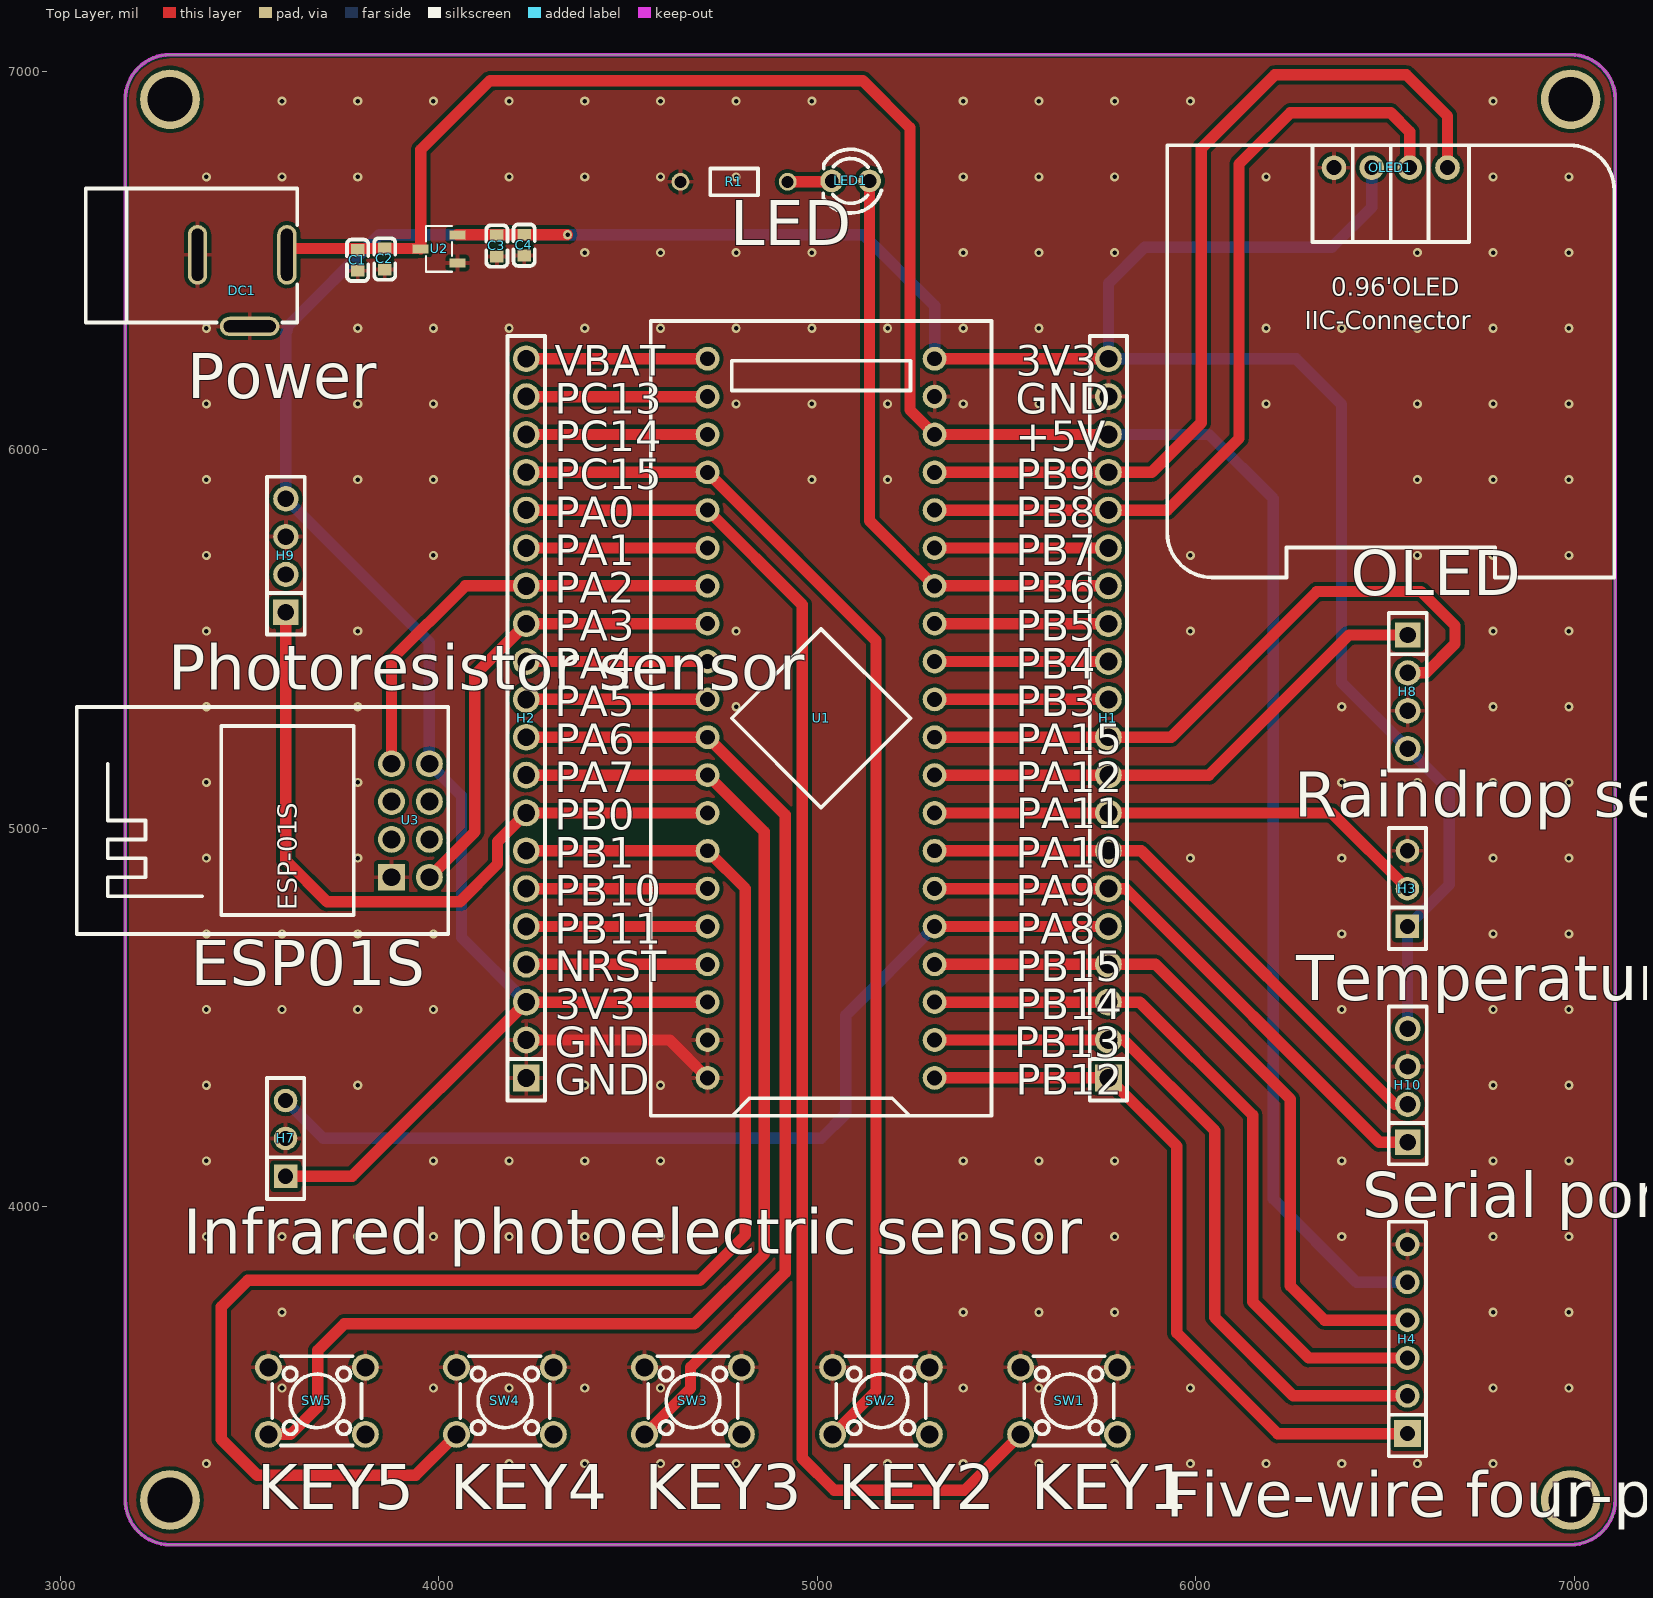
[diagram p0: Top Layer view]
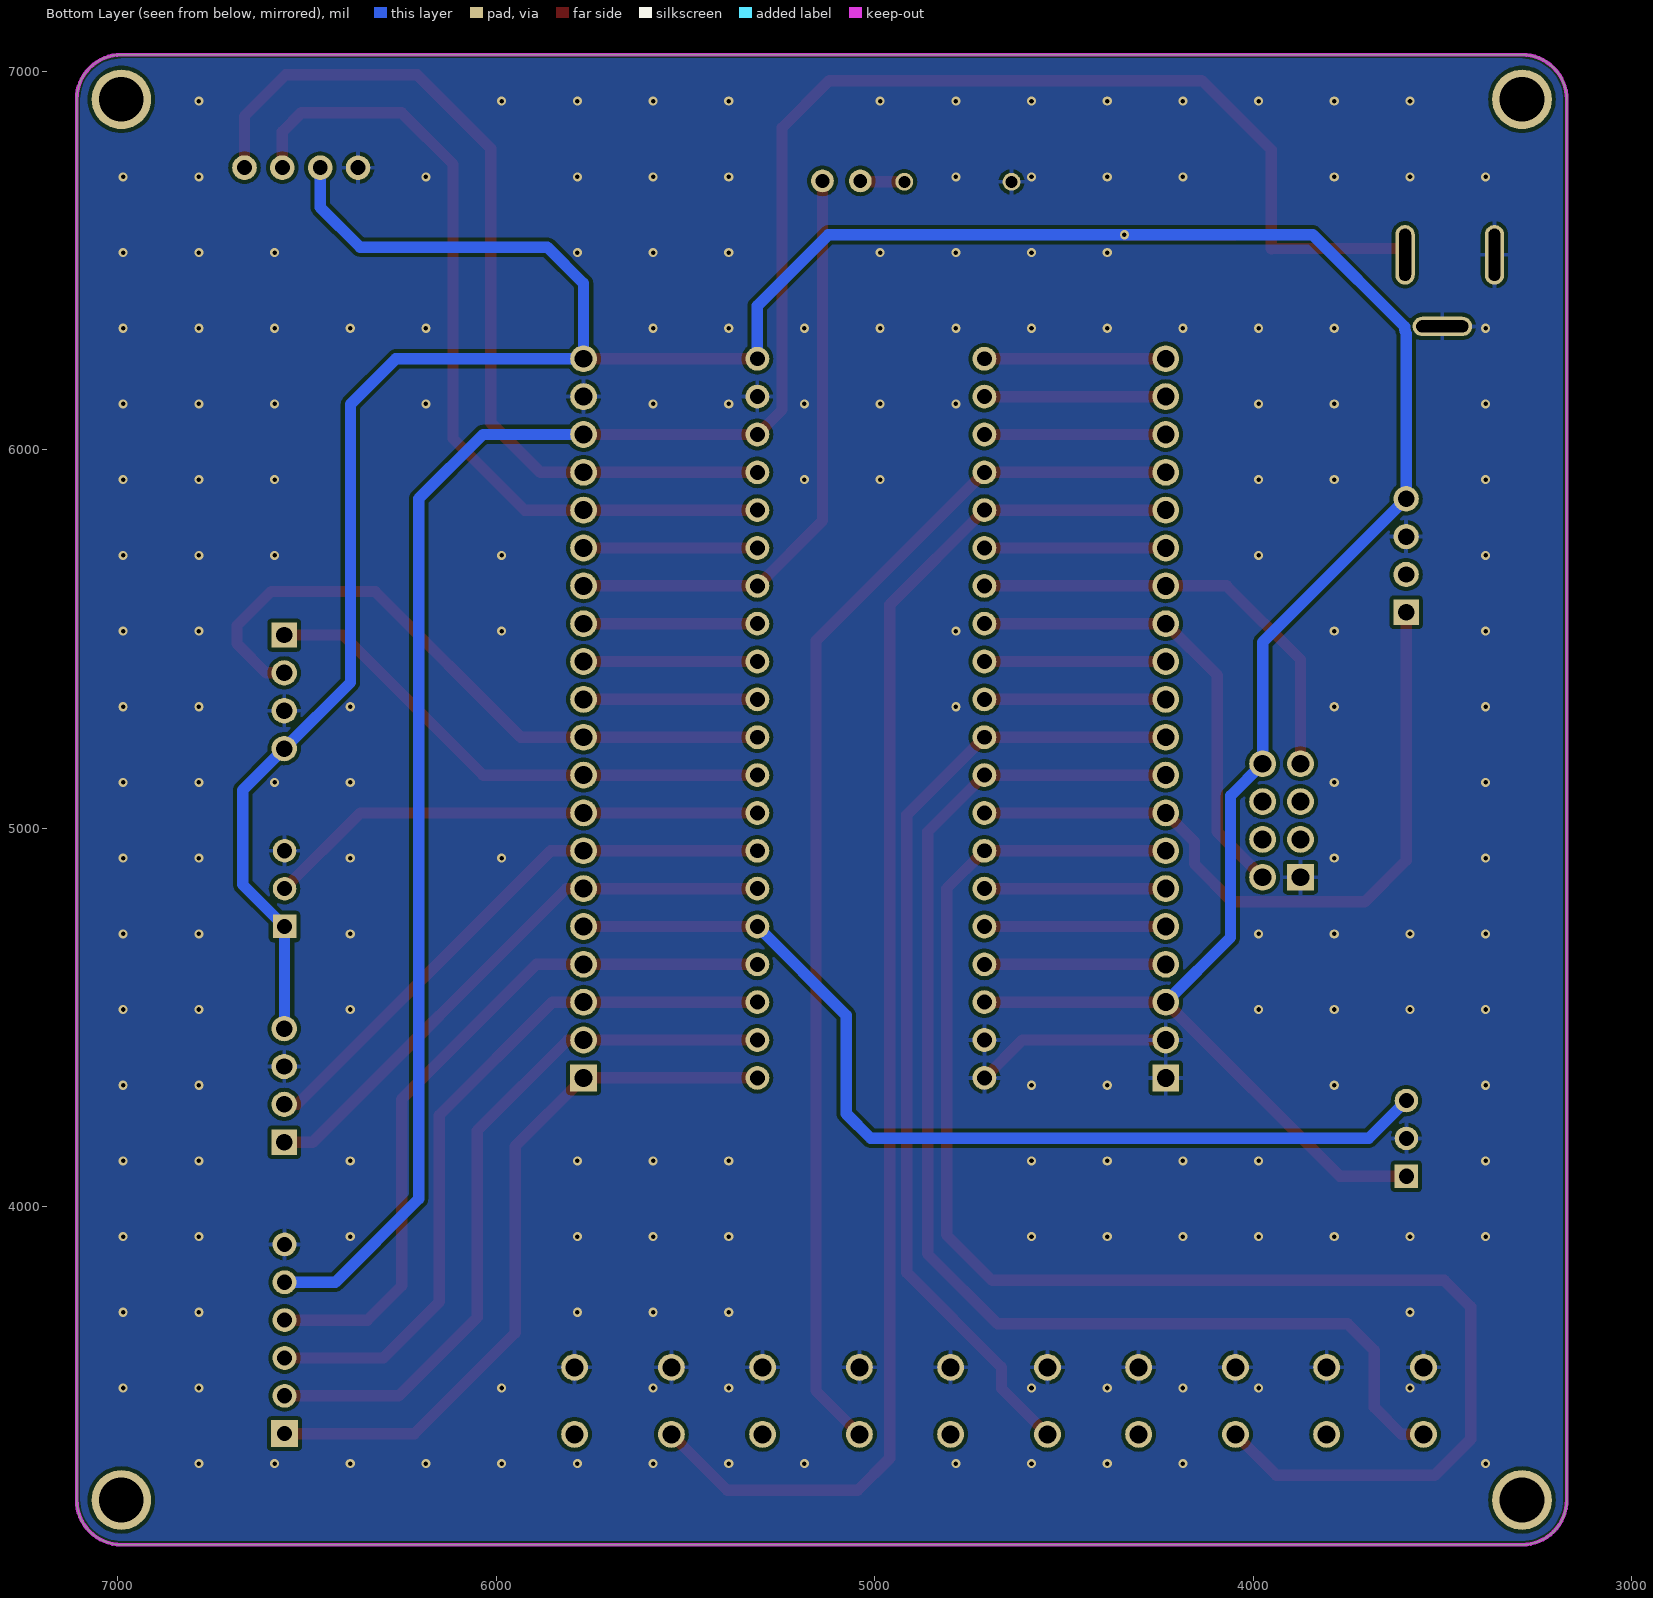
[diagram p1: Bottom Layer view, seen from below]
# Altium PCB MISC50760.pcbdoc
Units mil, origin at the board's own origin, x right, y up, seen from the top; angles counter-clockwise.
Board outline 3937.01 x 3937.01 mil, 2 copper layers (Top Layer, Bottom Layer), stack 62.206 mil thick; 24 components, 38 nets, 158 pads, 177 vias.

## Layer stack, top to bottom
Top Solder Mask Layer: solder mask 0.394, Dk 3.3
Top Layer: signal copper 1.379
Dielectric1: surface 59.449, FR4, Dk 4.5
Bottom Layer: signal copper 1.378
Bottom Solder Mask Layer: solder mask 0.394, Dk 3.3

## Board outline
3289.61,7043.5 ccw(c3289.61,6925.39) 3171.5,6925.39 3171.5,3224.61 ccw(c3289.61,3224.61) 3289.61,3106.5 6990.39,3106.5 ccw(c6990.39,3224.61) 7108.5,3224.61 7108.5,6925.39 ccw(c6990.39,6925.39) 6990.39,7043.5 3289.61,7043.5

## Design rules (kind name [scope] priority, off if disabled: settings)
BoardOutlineClearance copperThickness2oz_1 [All] p2 off: genericclearance=7.99 ignorepadtopadclearanceinfootprint=FALSE except(0: Arc-SplitContinuation Track-SplitContinuation SMDPad-SplitContinuation THPad-SplitContinuation Via-SplitContinuation Fill-SplitContinuation Region-SplitContinuation Poly-SplitContinuation Text-SplitContinuation Hole-SplitContinuation; 5.98: Arc-CutoutEdge Track-CutoutEdge SMDPad-CutoutEdge THPad-CutoutEdge Via-CutoutEdge Text-CutoutEdge; 6.9: Hole-OutlineEdge Hole-CutoutEdge; 10: Poly-OutlineEdge Poly-CutoutEdge; 11.81: Arc-OutlineEdge Track-OutlineEdge SMDPad-OutlineEdge THPad-OutlineEdge Via-OutlineEdge Fill-OutlineEdge Region-OutlineEdge Text-OutlineEdge Fill-CutoutEdge Region-CutoutEdge)
BoardOutlineClearance Plane_innerPlane_1 [All] p4 off: genericclearance=4.02 ignorepadtopadclearanceinfootprint=FALSE except(0: Arc-SplitContinuation Track-SplitContinuation SMDPad-SplitContinuation THPad-SplitContinuation Via-SplitContinuation Fill-SplitContinuation Region-SplitContinuation Poly-SplitContinuation Text-SplitContinuation Hole-SplitContinuation; 5.98: Arc-CutoutEdge Track-CutoutEdge SMDPad-CutoutEdge THPad-CutoutEdge Via-CutoutEdge Text-CutoutEdge; 6.9: Hole-OutlineEdge Hole-CutoutEdge; 10: Poly-OutlineEdge Poly-CutoutEdge; 11.81: Arc-OutlineEdge Track-OutlineEdge SMDPad-OutlineEdge THPad-OutlineEdge Via-OutlineEdge Fill-OutlineEdge Region-OutlineEdge Text-OutlineEdge Fill-CutoutEdge Region-CutoutEdge)
BoardOutlineClearance Copper_copperRegion_1 [All] p6 off: genericclearance=4.02 ignorepadtopadclearanceinfootprint=FALSE except(0: Arc-SplitContinuation Track-SplitContinuation SMDPad-SplitContinuation THPad-SplitContinuation Via-SplitContinuation Fill-SplitContinuation Region-SplitContinuation Poly-SplitContinuation Text-SplitContinuation Hole-SplitContinuation; 5.98: Arc-CutoutEdge Track-CutoutEdge SMDPad-CutoutEdge THPad-CutoutEdge Via-CutoutEdge Text-CutoutEdge; 6.9: Hole-OutlineEdge Hole-CutoutEdge; 10: Poly-OutlineEdge Poly-CutoutEdge; 11.81: Arc-OutlineEdge Track-OutlineEdge SMDPad-OutlineEdge THPad-OutlineEdge Via-OutlineEdge Fill-OutlineEdge Region-OutlineEdge Text-OutlineEdge Fill-CutoutEdge Region-CutoutEdge)
BoardOutlineClearance copperThickness1oz_1 [All] p8: genericclearance=4.02 ignorepadtopadclearanceinfootprint=FALSE except(0: Arc-SplitContinuation Track-SplitContinuation SMDPad-SplitContinuation THPad-SplitContinuation Via-SplitContinuation Fill-SplitContinuation Region-SplitContinuation Poly-SplitContinuation Text-SplitContinuation Hole-SplitContinuation; 5.98: Arc-CutoutEdge Track-CutoutEdge SMDPad-CutoutEdge THPad-CutoutEdge Via-CutoutEdge Text-CutoutEdge; 6.9: Hole-OutlineEdge Hole-CutoutEdge; 10: Poly-OutlineEdge Poly-CutoutEdge; 11.81: Arc-OutlineEdge Track-OutlineEdge SMDPad-OutlineEdge THPad-OutlineEdge Via-OutlineEdge Fill-OutlineEdge Region-OutlineEdge Text-OutlineEdge Fill-CutoutEdge Region-CutoutEdge)
Clearance copperThickness2oz [All] p1 off: gap=7.99 ignorepadtopadclearanceinfootprint=FALSE except(5.98: SMDPad-Track SMDPad-SMDPad THPad-Track SMDPad-THPad THPad-THPad Track-Via SMDPad-Via THPad-Via Via-Via Fill-SMDPad Region-SMDPad Fill-THPad Region-THPad Fill-Via Region-Via Fill-Fill Fill-Region Region-Region Arc-Track Arc-SMDPad Arc-THPad Arc-Via Fill-Arc Region-Arc Arc-Arc Text-Track SMDPad-Text Text-THPad Text-Via Fill-Text Region-Text Arc-Text Text-Text; 6.9: Hole-Track Hole-SMDPad Hole-THPad Hole-Via Fill-Hole Region-Hole Hole-Arc Hole-Text; 10: Poly-Track Poly-SMDPad Poly-THPad Poly-Via Poly-Fill Poly-Region Poly-Poly Poly-Arc Poly-Text Poly-Hole; 11.81: Fill-Track Region-Track)
Clearance Plane_innerPlane [All] p3 off: gap=4.02 ignorepadtopadclearanceinfootprint=FALSE except(5.98: SMDPad-Track SMDPad-SMDPad THPad-Track SMDPad-THPad THPad-THPad Track-Via SMDPad-Via THPad-Via Via-Via Fill-SMDPad Region-SMDPad Fill-THPad Region-THPad Fill-Via Region-Via Fill-Fill Fill-Region Region-Region Arc-Track Arc-SMDPad Arc-THPad Arc-Via Fill-Arc Region-Arc Arc-Arc Text-Track SMDPad-Text Text-THPad Text-Via Fill-Text Region-Text Arc-Text Text-Text; 6.9: Hole-Track Hole-SMDPad Hole-THPad Hole-Via Fill-Hole Region-Hole Hole-Arc Hole-Text; 10: Poly-Track Poly-SMDPad Poly-THPad Poly-Via Poly-Fill Poly-Region Poly-Poly Poly-Arc Poly-Text Poly-Hole; 11.81: Fill-Track Region-Track)
Clearance Copper_copperRegion [All] p5 off: gap=4.02 ignorepadtopadclearanceinfootprint=FALSE except(5.98: SMDPad-Track SMDPad-SMDPad THPad-Track SMDPad-THPad THPad-THPad Track-Via SMDPad-Via THPad-Via Via-Via Fill-SMDPad Region-SMDPad Fill-THPad Region-THPad Fill-Via Region-Via Fill-Fill Fill-Region Region-Region Arc-Track Arc-SMDPad Arc-THPad Arc-Via Fill-Arc Region-Arc Arc-Arc Text-Track SMDPad-Text Text-THPad Text-Via Fill-Text Region-Text Arc-Text Text-Text; 6.9: Hole-Track Hole-SMDPad Hole-THPad Hole-Via Fill-Hole Region-Hole Hole-Arc Hole-Text; 10: Poly-Track Poly-SMDPad Poly-THPad Poly-Via Poly-Fill Poly-Region Poly-Poly Poly-Arc Poly-Text Poly-Hole; 11.81: Fill-Track Region-Track)
Clearance copperThickness1oz [All] p7: gap=4.02 ignorepadtopadclearanceinfootprint=FALSE except(5.98: SMDPad-Track SMDPad-SMDPad THPad-Track SMDPad-THPad THPad-THPad Track-Via SMDPad-Via THPad-Via Via-Via Fill-SMDPad Region-SMDPad Fill-THPad Region-THPad Fill-Via Region-Via Fill-Fill Fill-Region Region-Region Arc-Track Arc-SMDPad Arc-THPad Arc-Via Fill-Arc Region-Arc Arc-Arc Text-Track SMDPad-Text Text-THPad Text-Via Fill-Text Region-Text Arc-Text Text-Text; 6.9: Hole-Track Hole-SMDPad Hole-THPad Hole-Via Fill-Hole Region-Hole Hole-Arc Hole-Text; 10: Poly-Track Poly-SMDPad Poly-THPad Poly-Via Poly-Fill Poly-Region Poly-Poly Poly-Arc Poly-Text Poly-Hole; 11.81: Fill-Track Region-Track)
DiffPairsRouting differentialPair [All] p1: maxlimit=6 minlimit=6 mostfreqgap=6 toplayer_minwidth=5 toplayer_prefwidth=10 toplayer_maxwidth=100 toplayer_mingap=6 toplayer_prefgap=6 toplayer_maxgap=6 bottomlayer_minwidth=5 bottomlayer_prefwidth=10 bottomlayer_maxwidth=100 bottomlayer_mingap=6 bottomlayer_prefgap=6 bottomlayer_maxgap=6 maxuncoupledlength=10
HoleToHoleClearance otherClearance [All] p1: gap=11.81 allowstackedmicrovias=TRUE
Length netLength [All] p1: minlimit=0 maxlimit=0
PasteMaskExpansion pasteMaskExpansion [All] p1: expansion=0
PlaneConnect innerPlane [All] p1: planeconnectstyle=Relief reliefexpansion=20 reliefentries=4 reliefconductorwidth=10 reliefairgap=10
PolygonConnect copperRegion [All] p1: connectstyle=Relief reliefconductorwidth=10 reliefentries=4 polygonreliefangle="90 Angle" airgapwidth=10 via.connectstyle=Relief via.reliefconductorwidth=10 via.reliefentries=4 via.polygonreliefangle="90 Angle" via.airgapwidth=10
RoutingVias viaSize [All] p1: holewidth=12.01 width=24.02 viastyle="Through Hole" minholewidth=11.81 minwidth=19.68 maxholewidth=248.03 maxwidth=393.7
SolderMaskExpansion solderMaskExpansion [IsVia] p1: expansion=-1000 istentingtop=TRUE
SolderMaskExpansion solderMaskExpansion [All] p2: expansion=2 istentingtop=FALSE
Width copperThickness2oz_2 [All] p1 off: maxlimit=100 minlimit=8 preferedwidth=10
Width copperThickness1oz_2 [All] p2: maxlimit=100 minlimit=5 preferedwidth=10

## Components (designator, comment, footprint, x,y, rotation, side; value= is the part's Value field where it differs from the comment)
C1 "10uF" C0603 3785.45,6500.1 r90 top
C2 "100nF" C0603 3856.99,6503.61 r90 top
C3 "10uF" C0603 4153.37,6538.01 r90 top
C4 "100nF" C0603 4225.45,6540.1 r90 top
DC1 "" DC-2.0 3475.44,6525.1 r180 top
H1 "" HDR-TH_20P-P2.54-V-F 5769.16,5290 r90 top
H2 "" HDR-TH_20P-P2.54-V-F 4230.95,5290 r90 top
H3 "" HDR-TH_3P-P2.54-V-F 6559.21,4840 r90 top
H4 "" HDR-TH_6P-P2.54-V-F 6559.21,3650 r90 top
H7 "" HDR-TH_3P-P2.54-V-F 3595,4180 r90 top
H8 "" HDR-TH_4P-P2.54-V-F 6560,5360 r270 top
H9 "" HDR-TH_4P-P2.54-V-F 3595.79,5720 r90 top
H10 "" HDR-TH_4P-P2.54-V-F 6560,4320 r90 top
LED1 "" LED_TH-3mm 5087.95,6709.8 r180 top
OLED1 "" 0.96OLED_4P 6515,6745 r0 top
R1 "220" Res_1/8W 4780,6710 r180 top
SW1 "" SW-TH_4P-L6.0-W6.0-P4.50-LS6.5 5665,3486.58 r0 top
SW2 "" SW-TH_4P-L6.0-W6.0-P4.50-LS6.5 5168.22,3486.58 r0 top
SW3 "" SW-TH_4P-L6.0-W6.0-P4.50-LS6.5 4671.43,3486.58 r0 top
SW4 "" SW-TH_4P-L6.0-W6.0-P4.50-LS6.5 4174.65,3486.58 r0 top
SW5 "" SW-TH_4P-L6.0-W6.0-P4.50-LS6.5 3677.86,3486.58 r0 top
U1 "STM32F103C8T6-Card" CONN-TH_L53.3-W22.9_STM32F103C8T6-CARD 5010,5290 r90 top
U2 "HT7333" SOT-23-3_L2.9-W1.6-P1.90-LS2.8-BR 4000.45,6530.1 r0 top
U3 "ESP-01S" WIFIM-TH_ESP-01S 3925,5020 r90 top

## Footprints (in the part's own frame and the unit in brackets; to place one, negate y for a bottom-side part, rotate by r counter-clockwise, add the part's x,y. Pads: shape width x height; smd on the part's side, far side on the other; paste and mask are expansions set on the pad)
0.96OLED_4P [mm]
  round 1.65 hole 1 copper offset 0,0: 1(-3.81,-0.001) 2(-1.27,0.002) 3(1.27,0.002) 4(3.81,0.002)
  silkscreen extent -15,-27.5 15,1.5
C0603 [mm]
  rect 0.8x0.9 smd: 1(-0.7,0) 2(0.7,0)
  silkscreen extent -1.39,-0.71 1.39,0.71
CONN-TH_L53.3-W22.9_STM32F103C8T6-CARD [mm]
  round 1.6 hole 1: 1(-24.13,-7.62) 2(-21.59,-7.62) 3(-19.05,-7.62) 4(-16.51,-7.62) 5(-13.97,-7.62) 6(-11.43,-7.62) 7(-8.89,-7.62) 8(-6.35,-7.62) 9(-3.81,-7.62) 10(-1.27,-7.62) 11(1.27,-7.62) 12(3.81,-7.62) 13(6.35,-7.62) 14(8.89,-7.62) 15(11.43,-7.62) 16(13.97,-7.62) 17(16.51,-7.62) 18(19.05,-7.62) 19(21.59,-7.62) 20(24.13,-7.62) 21(24.13,7.62) 22(21.59,7.62) 23(19.05,7.62) 24(16.51,7.62) 25(13.97,7.62) 26(11.43,7.62) 27(8.89,7.62) 28(6.35,7.62) 29(3.81,7.62) 30(1.27,7.62) 31(-1.27,7.62) 32(-3.81,7.62) 33(-6.35,7.62) 34(-8.89,7.62) 35(-11.43,7.62) 36(-13.97,7.62) 37(-16.51,7.62) 38(-19.05,7.62) 39(-21.59,7.62) 40(-24.13,7.62)
  silkscreen extent -26.67,-11.43 26.67,11.43
DC-2.0 [mil]
  oval 157.5x51.2 hole 31.5 slot 137.8 at 0 deg paste+0 mask+2: 2(-24.7,199.5)
  oval 51.2x157.5 hole 31.5 slot 137.8 at 90 deg paste+0 mask+2: 3(113.1,10.5) 4(-123.1,10.5)
  silkscreen extent -151,-165 408,190
HDR-TH_3P-P2.54-V-F [mil]
  rect 62x62 hole 40.16: 1(-100,0)
  round 62 hole 40.16: 2(0,0) 3(100,0)
  silkscreen extent -160,-49 160,49
HDR-TH_4P-P2.54-V-F [mm]
  rect 1.7x1.7 hole 1.1: 1(-3.81,0)
  round 1.7 hole 1.1: 2(-1.27,0) 3(1.27,0) 4(3.81,0)
  silkscreen extent -5.29,-1.27 5.29,1.27
HDR-TH_6P-P2.54-V-F [mm]
  rect 1.8x1.8 hole 1.02: 1(-6.35,0)
  round 1.6 hole 1.02: 2(-3.81,0) 3(-1.27,0) 4(1.27,0) 5(3.81,0) 6(6.35,0)
  silkscreen extent -7.87,-1.25 7.87,1.25
HDR-TH_20P-P2.54-V-F [mm]
  rect 1.8x1.8 hole 1.2: 1(-24.13,0)
  round 1.8 hole 1.2: 2(-21.59,0) 3(-19.05,0) 4(-16.51,0) 5(-13.97,0) 6(-11.43,0) 7(-8.89,0) 8(-6.35,0) 9(-3.81,0) 10(-1.27,0) 11(1.27,0) 12(3.81,0) 13(6.35,0) 14(8.89,0) 15(11.43,0) 16(13.97,0) 17(16.51,0) 18(19.05,0) 19(21.59,0) 20(24.13,0)
  silkscreen extent -25.65,-1.25 25.65,1.25
LED_TH-3mm [mil]
  round 60 hole 36 paste+0 mask+2: 1(-50,0) 2(50,0)
  silkscreen extent -81,-84 72,85
Res_1/8W [mil]
  round 47.2 hole 31.5 paste+0 mask+2: 1(-141.7,2.48) 2(141.7,2.48)
  silkscreen extent -63,-33 63,38
SOT-23-3_L2.9-W1.6-P1.90-LS2.8-BR [mm]
  rect 1.07x0.6 smd: 1(1.235,-0.95) 2(1.235,0.95) 3(-1.235,0)
  silkscreen extent -0.88,-1.54 0.88,1.54
SW-TH_4P-L6.0-W6.0-P4.50-LS6.5 [mm]
  round 1.8 hole 1.2: 1(-3.25,2.25) 2(3.25,2.25) 3(-3.25,-2.25) 4(3.25,-2.25)
  silkscreen extent -3,-3 3,3
WIFIM-TH_ESP-01S [mm]
  rect 1.8x1.8 hole 1.2: 1(-3.81,1.27)
  round 1.8 hole 1.2: 2(-1.27,1.27) 3(1.27,1.27) 4(3.81,1.27) 5(3.81,-1.27) 6(1.27,-1.27) 7(-1.27,-1.27) 8(-3.81,-1.27)
  silkscreen extent -7.62,-2.54 7.62,22.4

## Free pads (board coordinates)
  round 157.48 hole 118.11: 1(3289.61,6925.39) 1(3289.61,3224.61) 1(6990.39,6925.39) 1(6990.39,3224.61)

## Via types
v1: diameter 24.02, hole 12, Top Layer to Bottom Layer, 177 vias

## Nets (pads, with @x,y where several pads share a name; then routed paths per layer and width w, separated by ;. In a path a pad name is that pad's centre, name@x,y a point inside that pad or via, vN(x,y) a via of type N, cw(c..) or ccw(c..) an arc to the next point about the centre after c; other vN are vias at no path point)
$1N17011: LED1.2 R1.1 | length 117.2
  Top Layer w30: R1.1 5035.67,6707.52 LED1.2
+5V: C1.2 C2.2 DC1.4 H1.18 H4.5 U1.18 U2.3 | length 6140.8
  Top Layer w30: DC1.4 3615.11,6531.17 C2.2 3950.75,6531.17 U2.3 3951.82,6791.82 4135,6975 5120,6975 5245,6850 5245,6105 U1.18 H1.18
  Bottom Layer w30: H1.18 6035,6040 6205,5870 6205,4020 6425,3800 H4.5
GND: C1.1 C2.1 C3.1 C4.1 DC1.2 DC1.3 H1.19 H2.1 H2.2 H3.3 H4.6 H7.2 H8.3 H9.3 H10.3 OLED1.1 R1.2 SW1.1 SW1.2 SW2.1 SW2.2 SW3.1 SW3.2 SW4.1 SW4.2 SW5.1 SW5.2 U1.19 U1.39 U1.40 U2.1 U3.1 | length 520.5
  Top Layer w30: H2.2 4610,4440 U1.40
  other v1: 3385.6,3320.6 4185.6,3320.6 4385.6,3320.6 4585.6,3320.6 4785.6,3320.6 5185.6,3320.6 5385.6,3320.6 5585.6,3320.6 5785.6,3320.6 5985.6,3320.6 6185.6,3320.6 6385.6,3320.6 6585.6,3320.6 6785.6,3320.6 3585.6,3520.6 3985.6,3520.6 4185.6,3520.6 4385.6,3520.6 4585.6,3520.6 5385.6,3520.6 5585.6,3520.6 5985.6,3520.6 6785.6,3520.6 6985.6,3520.6 3585.6,3720.6 5385.6,3720.6 5585.6,3720.6 5785.6,3720.6 6785.6,3720.6 6985.6,3720.6 3385.6,3920.6 3585.6,3920.6 3785.6,3920.6 3985.6,3920.6 4185.6,3920.6 4385.6,3920.6 4585.6,3920.6 5385.6,3920.6 5585.6,3920.6 5785.6,3920.6 6385.6,3920.6 6785.6,3920.6 6985.6,3920.6 3385.6,4120.6 3985.6,4120.6 4185.6,4120.6 4385.6,4120.6 4585.6,4120.6 5385.6,4120.6 5585.6,4120.6 5785.6,4120.6 6385.6,4120.6 6785.6,4120.6 6985.6,4120.6 3385.6,4320.6 3785.6,4320.6 4385.6,4320.6 4585.6,4320.6 6785.6,4320.6 6985.6,4320.6 3385.6,4520.6 3585.6,4520.6 3785.6,4520.6 3985.6,4520.6 6385.6,4520.6 6785.6,4520.6 6985.6,4520.6 3385.6,4720.6 3585.6,4720.6 3785.6,4720.6 3985.6,4720.6 6385.6,4720.6 6785.6,4720.6 6985.6,4720.6 3385.6,4920.6 3785.6,4920.6 5985.6,4920.6 6385.6,4920.6 6785.6,4920.6 6985.6,4920.6 3385.6,5120.6 3785.6,5120.6 6385.6,5120.6 6585.6,5120.6 6785.6,5120.6 6985.6,5120.6 3385.6,5320.6 3785.6,5320.6 4785.6,5320.6 6385.6,5320.6 6785.6,5320.6 6985.6,5320.6 3385.6,5520.6 3785.6,5520.6 4785.6,5520.6 5985.6,5520.6 6785.6,5520.6 6985.6,5520.6 3385.6,5720.6 3985.6,5720.6 5985.6,5720.6 6585.6,5720.6 6785.6,5720.6 6985.6,5720.6 3385.6,5920.6 3785.6,5920.6 3985.6,5920.6 4985.6,5920.6 5185.6,5920.6 6585.6,5920.6 6785.6,5920.6 6985.6,5920.6 3385.6,6120.6 3785.6,6120.6 3985.6,6120.6 4785.6,6120.6 4985.6,6120.6 5185.6,6120.6 5385.6,6120.6 5585.6,6120.6 6185.6,6120.6 6585.6,6120.6 6785.6,6120.6 6985.6,6120.6 3385.6,6320.6 3785.6,6320.6 3985.6,6320.6 4185.6,6320.6 4385.6,6320.6 4585.6,6320.6 4785.6,6320.6 4985.6,6320.6 5185.6,6320.6 5385.6,6320.6 5585.6,6320.6 6185.6,6320.6 6385.6,6320.6 6585.6,6320.6 6785.6,6320.6 6985.6,6320.6 4385.6,6520.6 4585.6,6520.6 4785.6,6520.6 4985.6,6520.6 5385.6,6520.6 5585.6,6520.6 5785.6,6520.6 6585.6,6520.6 6785.6,6520.6 6985.6,6520.6 3385.6,6720.6 3585.6,6720.6 3785.6,6720.6 4185.6,6720.6 4385.6,6720.6 4585.6,6720.6 4785.6,6720.6 5385.6,6720.6 5585.6,6720.6 5785.6,6720.6 6185.6,6720.6 6785.6,6720.6 6985.6,6720.6 3585.6,6920.6 3785.6,6920.6 3985.6,6920.6 4185.6,6920.6 4385.6,6920.6 4585.6,6920.6 4785.6,6920.6 4985.6,6920.6 5385.6,6920.6 5585.6,6920.6 5785.6,6920.6 5985.6,6920.6 6785.6,6920.6
NRST: H2.4 U1.37 | length 479
  Top Layer w30: H2.4 U1.37
PA0: H2.16 SW1.3 U1.25 | length 3761.2
  Top Layer w30: H2.16 U1.25 4960,5590 4960,3335 5045,3250 5389.05,3250 SW1.3
PA1: H2.15 U1.26 | length 479
  Top Layer w30: H2.15 U1.26
PA2: H2.14 U1.27 U3.4 | length 1190.8
  Top Layer w30: U3.4 3875,5445 4070,5640 H2.14 U1.27
PA3: H2.13 U1.28 U3.8 | length 1255.1
  Top Layer w30: U3.8 4095,4990 4095,5404.05 H2.13 U1.28
PA4: H2.12 U1.29 | length 479
  Top Layer w30: H2.12 U1.29
PA5: H2.11 U1.30 | length 479
  Top Layer w30: H2.11 U1.30
PA6: H2.10 SW3.3 U1.31 | length 2559.9
  Top Layer w30: H2.10 U1.31 4915,5035 4915,3825 4665,3575 4665,3519.52 SW3.3
PA7: H2.9 SW5.3 U1.32 | length 3401.7
  Top Layer w30: SW5.3 3608,3398 3680,3470 3680,3620 3750,3690 4675,3690 4860,3875 4860,4990 U1.32 H2.9
PA8: H1.5 H7.3 U1.5 | length 2599.8
  Top Layer w30: U1.5 H1.5
  Bottom Layer w30: H7.3 3695,4180 5010,4180 5075,4245 5075,4505 U1.5
PA9: H1.6 H10.1 U1.6 | length 1527.5
  Top Layer w30: U1.6 H1.6 5814.59,4840 6484.59,4170 H10.1
PA10: H1.7 H10.2 U1.7 | length 1527.5
  Top Layer w30: U1.7 H1.7 5856.01,4940 6526.01,4270 H10.2
PA11: H1.8 H3.2 U1.8 | length 1332.1
  Top Layer w30: U1.8 H1.8 6359.21,5040 H3.2
PA12: H1.9 H8.1 U1.9 | length 1403.3
  Top Layer w30: U1.9 H1.9 6035,5140 6405,5510 H8.1
PA15: H1.10 H8.2 U1.10 | length 1776.7
  Top Layer w30: U1.10 H1.10 5935,5240 6320,5625 6595,5625 6685,5535 6685,5486.89 6608.11,5410 H8.2
PB0: H2.8 H9.1 U1.33 | length 1947.2
  Top Layer w30: H9.1 3595.79,4914.21 3705,4805 4055,4805 4155,4905 4155,4964.05 H2.8 U1.33
PB1: H2.7 SW4.3 U1.34 | length 4055
  Top Layer w30: SW4.3 3938.7,3290 3520,3290 3425,3385 3425,3735 3495,3805 4690,3805 4810,3925 4810,4840 U1.34 H2.7
PB3: H1.11 U1.11 | length 459.2
  Top Layer w30: U1.11 H1.11
PB4: H1.12 U1.12 | length 459.2
  Top Layer w30: U1.12 H1.12
PB5: H1.13 U1.13 | length 459.2
  Top Layer w30: U1.13 H1.13
PB6: H1.14 LED1.1 U1.14 | length 1600.2
  Top Layer w30: LED1.1 5137.95,5812.05 U1.14 H1.14
PB7: H1.15 U1.15 | length 459.2
  Top Layer w30: U1.15 H1.15
PB8: H1.16 OLED1.3 U1.16 | length 2230.3
  Top Layer w30: U1.16 H1.16 5925,5840 6114.29,6029.29 6114.29,6754.29 6250,6890 6515,6890 6565,6840 OLED1.3@6565,6745.05
PB9: H1.17 OLED1.4 U1.17 | length 2396
  Top Layer w30: U1.17 H1.17 5883.58,5940 6014.29,6070.71 6014.29,6795.71 6208.58,6990 6556.42,6990 6665,6881.42 OLED1.4@6665,6745.05
PB10: H2.6 U1.35 | length 479
  Top Layer w30: H2.6 U1.35
PB11: H2.5 U1.36 | length 479
  Top Layer w30: H2.5 U1.36
PB12: H1.1 H4.1 U1.1 | length 1927.6
  Top Layer w30: U1.1 H1.1 5950,4159.16 5950,3665.74 6215.74,3400 H4.1
PB13: H1.2 H4.2 U1.2 | length 1927.6
  Top Layer w30: U1.2 H1.2 5810.58,4440 6050,4200.58 6050,3707.16 6257.16,3500 H4.2
PB14: H1.3 H4.3 U1.3 | length 1927.6
  Top Layer w30: U1.3 H1.3 5852,4540 6150,4242 6150,3748.58 6298.58,3600 H4.3
PB15: H1.4 H4.4 U1.4 | length 1927.6
  Top Layer w30: U1.4 H1.4 5893.42,4640 6250,4283.42 6250,3790 6340,3700 H4.4
PC13: H2.19 U1.22 | length 479
  Top Layer w30: H2.19 U1.22
PC14: H2.18 U1.23 | length 479
  Top Layer w30: H2.18 U1.23
PC15: H2.17 SW2.3 U1.24 | length 3252.9
  Top Layer w30: H2.17 U1.24 5155,5495 5155,3512.73 SW2.3
VBAT: H2.20 U1.21 | length 479
  Top Layer w30: H2.20 U1.21
VCC: C3.2 C4.2 H1.20 H2.3 H3.1 H7.1 H8.4 H9.4 H10.4 OLED1.2 U1.20 U1.38 U2.2 U3.5 | length 9695.7
  Top Layer w30: H7.1 3770.95,4080 H2.3 U1.38 ; U2.2 4225.29,6567.5 C4.2 v1(4340,6567.66) ; U1.20 H1.20
  Bottom Layer w30: H2.3 4060,4710.95 4060,5085 U3.5 3975,5490.79 H9.4 3595.79,6306.51 ccw(c3553.29,6325.6) 3599.87,6324.87 3842.66,6567.66 v1(4340,6567.66) 5122.34,6567.66 5310,6380 U1.20 ; OLED1.2@6465,6745.05 6465,6640 6360,6535 5865,6535 5769.16,6439.16 H1.20 6265,6240 6385,6120 6385,5385 H8.4 6670,5100 6670,4850.79 H3.1 6559.21,4470.79 H10.4
pads on no net: H9.2 SW1.4 SW2.4 SW3.4 SW4.4 SW5.4 U3.2 U3.3 U3.6 U3.7

## Polygon pours and split planes (outlines as drawn)
GND on Bottom Layer (solid, remove dead copper, pour order 2): 3100,7165 3100,3000 7275,3000 7275,7165
GND on Top Layer (solid, remove dead copper, pour order 0): 3000,7145 3000,3075 7385,3075 7385,7145

## Keep-outs
Board Outline Layer:
  the board outline again, w10

## Silkscreen, mask and mechanical layers (free items; w line width, h text height)
Top Silkscreen Layer:
  text "LED" at 4770,6540 h120
  text "VBAT" at 4305.95,6195 h80
  text "3V3" at 5524.16,6195 h80
  text "Power" at 3335,6135 h120
  text "PC13" at 4305.95,6095 h80
  text "GND" at 5524.16,6095 h80
  text "PC14" at 4305.95,5995 h80
  text "+5V" at 5524.16,5995 h80
  text "PC15" at 4305.95,5895 h80
  text "PB9" at 5524.16,5895 h80
  text "PA0" at 4305.95,5795 h80
  text "PB8" at 5524.16,5795 h80
  text "PA1" at 4305.95,5695 h80
  text "PB7" at 5524.16,5695 h80
  text "OLED" at 6410,5615 h120
  text "PA2" at 4305.95,5595 h80
  text "PB6" at 5524.16,5595 h80
  text "PA3" at 4305.95,5495 h80
  text "PB5" at 5524.16,5495 h80
  text "PA4" at 4305.95,5395 h80
  text "PB4" at 5524.16,5395 h80
  text "Photoresistor sensor" at 3285,5365 h120
  text "PA5" at 4305.95,5295 h80
  text "PB3" at 5524.16,5295 h80
  text "PA6" at 4305.95,5195 h80
  text "PA15" at 5524.16,5195 h80
  text "PA7" at 4305.95,5095 h80
  text "PA12" at 5524.16,5095 h80
  text "Raindrop sensor" at 6260,5030 h120
  text "PA11" at 5525.95,5000 h80
  text "PB0" at 4305.95,4995 h80
  text "PB1" at 4305.95,4895 h80
  text "PA10" at 5524.16,4895 h80
  text "PB10" at 4305.95,4795 h80
  text "PA9" at 5524.16,4795 h80
  text "PB11" at 4305.95,4695 h80
  text "PA8" at 5524.16,4695 h80
  text "NRST" at 4305.95,4595 h80
  text "PB15" at 5524.16,4595 h80
  text "ESP01S" at 3345,4585 h120
  text "Temperature and humidity sensor" at 6265,4545 h120
  text "3V3" at 4305.95,4495 h80
  text "PB14" at 5524.16,4495 h80
  text "GND" at 4305.95,4395 h80
  text "PB13" at 5520.95,4395 h80
  text "GND" at 4305.95,4295 h80
  text "PB12" at 5524.16,4295 h80
  text "Serial port" at 6439.21,3972.37 h120
  text "Infrared photoelectric sensor" at 3325,3875 h120
  text "KEY5" at 3520,3200 h120
  text "KEY4" at 4030.38,3200 h120
  text "KEY3" at 4544.25,3200 h120
  text "KEY2" at 5054.62,3200 h120
  text "KEY1" at 5565,3200 h120
  text "Five-wire four-phase stepper motor" at 5920,3180 h120